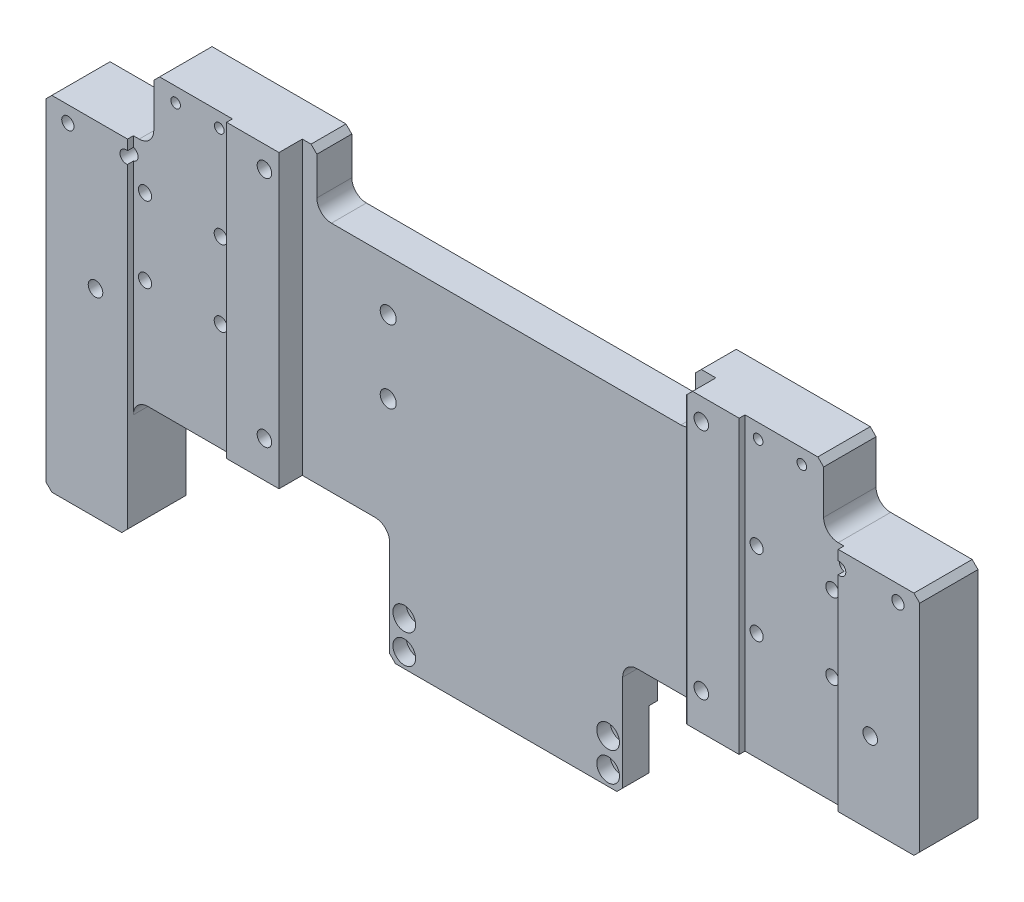
SolidWorks part; units mm, degrees
ref_plane "前视基准面" through (0, 0, 0) normal (0, 0, 1) x (1, 0, 0)
ref_plane "上视基准面" through (0, 0, 0) normal (0, 1, 0) x (1, 0, 0)
ref_plane "右视基准面" through (0, 0, 0) normal (1, 0, 0) x (0, 0, -1)
sketch "草图1" plane through (0, 0, 0) normal (0, 0, 1) x (1, 0, 0)
  line L1 (-150, -50) -> (150, -50)
  line L2 (-150, -50) -> (-150, 50)
  line L3 (-150, 50) -> (150, 50)
  line L4 (150, -50) -> (150, 50)
  line L5 (-150, -50) -> (150, 50) construction
  line L6 (-150, 50) -> (150, -50) construction
  point P0 (0, 0)
  dimension "D1" = 300
  dimension "D2" = 100
extrude "凸台-拉伸1" add sketch "草图1" along normal blind 20 contours L3 L4 L1 L2
chamfer "倒角1" distance 2 angle 45 3 edges at (-150, 50, 10) (150, 50, 10) (150, -50, 10)
sketch "草图2" plane through (0, -50, 0) normal (0, -1, 0) x (1, 0, 0)
  line L0 (-150, 20) -> (148, 20) construction
  line L1 (-122, 20) -> (-88, 20)
  line L2 (-122, 20) -> (-122, 18)
  line L3 (-122, 18) -> (-88, 18)
  line L4 (-88, 20) -> (-88, 18)
  line L6 (0, 0) -> (0, 81.6409) construction
  line L7 (88, 20) -> (88, 18)
  line L8 (122, 18) -> (88, 18)
  line L9 (122, 20) -> (122, 18)
  line L10 (122, 20) -> (88, 20)
  line L11 (-150, 20) -> (-150, 0) construction
  dimension "D1" = 34
  dimension "D2" = 28
  dimension "D3" = 2
extrude "切除-拉伸1" cut sketch "草图2" against normal through all
sketch "草图3" plane through (0, -50, 0) normal (0, -1, 0) x (1, 0, 0)
  line L5 (-88, 20) -> (88, 20) construction
  line L6 (-70, 20) -> (70, 20)
  line L7 (-70, 20) -> (-70, 12)
  line L8 (-70, 12) -> (70, 12)
  line L9 (70, 20) -> (70, 12)
  line L10 (0, 0) -> (0, 35.5532) construction
  dimension "D2" = 140
  dimension "D3" = 8
extrude "切除-拉伸2" cut sketch "草图3" against normal through all
sketch "草图4" plane through (0, 0, 0) normal (0, 0, -1) x (-1, 0, 0)
  line L0 (150, -50) -> (-148, -50) construction
  line L1 (-40, -50) -> (40, -50)
  line L2 (-40, -50) -> (-40, -90)
  line L3 (-40, -90) -> (40, -90)
  line L4 (40, -50) -> (40, -90)
  line L5 (0, 0) -> (0, -116.0992) construction
  dimension "D1" = 80
  dimension "D2" = 40
extrude "凸台-拉伸2" add sketch "草图4" against normal up to surface (12 mm away) up to face at (0, 0, 12)
fillet "圆角1" radius 5 2 edges at (40, -50, 6) (-40, -50, 6)
sketch "草图5" plane through (40, 0, 0) normal (1, 0, 0) x (0, 0, -1)
  line L1 (-3, -90) -> (0, -90)
  line L2 (-3, -90) -> (-3, -68)
  line L3 (-3, -68) -> (0, -68)
  line L4 (0, -90) -> (0, -68)
  line L5 (0, -55) -> (0, -90) construction
  line L6 (-12, -90) -> (0, -90) construction
  dimension "D1" = 22
  dimension "D3" = 3
extrude "切除-拉伸3" cut sketch "草图5" against normal through all
chamfer "倒角2" distance 2 angle 45 2 edges at (-40, -90, 7.5) (40, -90, 7.5)
sketch "草图6" plane through (0, 0, 0) normal (0, 0, -1) x (-1, 0, 0)
  line L1 (-65, 50) -> (65, 50)
  line L2 (-65, 50) -> (-65, 30)
  line L3 (-65, 30) -> (65, 30)
  line L4 (65, 50) -> (65, 30)
  line L5 (148, 50) -> (-148, 50) construction
  point P5 (0, 50)
  dimension "D1" = 20
  dimension "D2" = 130
extrude "切除-拉伸4" cut sketch "草图6" against normal through all
fillet "圆角2" radius 5 2 edges at (65, 30, 6) (-65, 30, 6)
sketch "草图9" plane through (0, 0, 0) normal (0, 0, -1) x (-1, 0, 0)
  line L0 (150, -50) -> (45, -50) construction
  line L1 (150, -50) -> (150, 48) construction
  line L2 (0, 0) -> (0, 75.4355) construction
  point P0 (133, -22)
  point P14 (-133, -22)
  dimension "D1" = 28
  dimension "D2" = 17
hole_wizard "M6 螺纹孔1" positions "草图9" profile "草图8" tap size "M6" standard "GB" end condition through all
sketch "草图8" plane through (-133, -22, 0) normal (1, 0, 0) x (0, 1, 0)
  line L0 (0, 0) -> (0, 20)
  line L1 (0, 20) -> (2.5, 20)
  line L2 (2.5, 20) -> (2.5, 0)
  line L5 (2.5, 0) -> (0, 0)
  line L11 (0, -6.35) -> (0, 107.95) construction
  dimension "通孔螺纹孔钻头直径" = 5
  dimension "通孔螺纹孔钻头深度" = 20
cosmetic thread "孔螺纹线1" parameters "D2"=6
cosmetic thread "孔螺纹线2" parameters "D2"=6
sketch "草图10" plane through (0, 0, 0) normal (0, 0, -1) x (-1, 0, 0)
  line L0 (150, -50) -> (150, 48) construction
  line L1 (150, 50) -> (115, 50)
  line L2 (150, 50) -> (150, 28)
  line L3 (150, 28) -> (115, 28)
  line L4 (115, 50) -> (115, 28)
  line L5 (148, 50) -> (65, 50) construction
  line L6 (0, 0) -> (0, 101.2863) construction
  line L7 (-115, 50) -> (-115, 28)
  line L8 (-150, 28) -> (-115, 28)
  line L9 (-150, 50) -> (-150, 28)
  line L10 (-150, 50) -> (-115, 50)
  dimension "D1" = 35
  dimension "D2" = 22
extrude "切除-拉伸5" cut sketch "草图10" against normal through all
chamfer "倒角3" distance 2 angle 45 5 edges at (150, 28, 10) (115, 50, 9) (70, 50, 16) (-115, 50, 9) (-150, 28, 10)
fillet "圆角3" radius 5 2 edges at (115, 28, 9) (-115, 28, 9)
sketch "草图13" plane through (0, 0, 0) normal (0, 0, -1) x (-1, 0, 0)
  point P0 (40.5, 12.5)
  point P3 (40.5, -12.5)
hole_wizard "M5 六角圆柱头螺钉的柱形沉头孔1" positions "草图13" profile "草图12" counterbore size "M5" standard "GB" end condition through all
sketch "草图12" plane through (-40.5, 12.5, 0) normal (1, 0, 0) x (0, 1, 0)
  line L0 (0, 0) -> (0, 20)
  line L1 (0, 20) -> (2.75, 20)
  line L3 (2.75, 20) -> (2.75, 5.7)
  line L4 (2.75, 5.7) -> (5, 5.7)
  line L5 (5, 5.7) -> (5, 0)
  line L7 (5, 0) -> (0, 0)
  line L11 (0, -6.35) -> (0, 107.95) construction
  dimension "通孔孔直径" = 5.5
  dimension "通孔孔深度" = 20
  dimension "柱形沉头孔直径" = 10
  dimension "柱形沉头孔深度" = 5.7
sketch "草图16" plane through (0, 0, 0) normal (0, 0, -1) x (-1, 0, 0)
  line L0 (0, 0) -> (0, 67.4868) construction
  point P0 (92, 13)
  point P3 (118, 13)
  point P6 (118, -13)
  point P9 (92, -13)
  point P19 (-92, -13)
  point P20 (-118, -13)
  point P21 (-118, 13)
  point P22 (-92, 13)
hole_wizard "M4 六角圆柱头螺钉的柱形沉头孔1" positions "草图16" profile "草图15" counterbore size "M4" standard "GB" end condition through all
sketch "草图15" plane through (-92, 13, 0) normal (1, 0, 0) x (0, 1, 0)
  line L0 (0, 0) -> (0, 20)
  line L1 (0, 20) -> (2.25, 20)
  line L3 (2.25, 20) -> (2.25, 4.6)
  line L4 (2.25, 4.6) -> (4, 4.6)
  line L5 (4, 4.6) -> (4, 0)
  line L7 (4, 0) -> (0, 0)
  line L11 (0, -6.35) -> (0, 107.95) construction
  dimension "通孔孔直径" = 4.5
  dimension "通孔孔深度" = 20
  dimension "柱形沉头孔直径" = 8
  dimension "柱形沉头孔深度" = 4.6
sketch "草图19" plane through (0, 0, 0) normal (0, 0, -1) x (-1, 0, 0)
  line L0 (0, 0) -> (0, 54.9806) construction
  point P0 (75, 42.5)
  point P3 (75, -37.5)
  point P12 (-75, -37.5)
  point P13 (-75, 42.5)
hole_wizard "M6 螺纹孔2" positions "草图19" profile "草图18" tap size "M6" standard "GB" end condition through all
sketch "草图18" plane through (-75, 42.5, 0) normal (1, 0, 0) x (0, 1, 0)
  line L0 (0, 0) -> (0, 20)
  line L1 (0, 20) -> (2.5, 20)
  line L2 (2.5, 20) -> (2.5, 0)
  line L5 (2.5, 0) -> (0, 0)
  line L11 (0, -6.35) -> (0, 107.95) construction
  dimension "通孔螺纹孔钻头直径" = 5
  dimension "通孔螺纹孔钻头深度" = 20
cosmetic thread "孔螺纹线3" parameters "D2"=6
cosmetic thread "孔螺纹线4" parameters "D2"=6
cosmetic thread "孔螺纹线5" parameters "D2"=6
cosmetic thread "孔螺纹线6" parameters "D2"=6
sketch "草图22" plane through (0, 0, 0) normal (0, 0, -1) x (-1, 0, 0)
  line L0 (0, 0) -> (0, 50.8482) construction
  point P0 (19.5, 20)
  point P3 (19.5, -10)
  point P11 (-19.5, -10)
  point P12 (-19.5, 20)
hole_wizard "M3 螺纹孔1" positions "草图22" profile "草图21" tap size "M3" standard "GB"
sketch "草图21" plane through (-19.5, 20, 0) normal (1, 0, 0) x (0, 1, 0)
  line L0 (0, 0) -> (0, 8.2511)
  line L1 (0, 8.2511) -> (1.25, 7.5)
  line L2 (1.25, 7.5) -> (1.25, 0)
  line L5 (1.25, 0) -> (0, 0)
  line L10 (0, 8.2511) -> (-1.25, 7.5) construction
  line L11 (0, -6.35) -> (0, 107.95) construction
  dimension "螺纹孔钻头直径" = 2.5
  dimension "螺纹孔钻头深度" = 7.5
  dimension "导头角度" = 118
cosmetic thread "孔螺纹线7" parameters "D1"=6, "D2"=3
cosmetic thread "孔螺纹线8" parameters "D1"=6, "D2"=3
cosmetic thread "孔螺纹线9" parameters "D1"=6, "D2"=3
cosmetic thread "孔螺纹线10" parameters "D1"=6, "D2"=3
sketch "草图25" plane through (0, 0, 0) normal (0, 0, -1) x (-1, 0, 0)
  line L0 (0, 0) -> (0, 56.662) construction
  point P0 (-142.5, 22.5)
  point P3 (-122.5, 22.5)
  point P12 (122.5, 22.5)
  point P13 (142.5, 22.5)
hole_wizard "M5 螺纹孔1" positions "草图25" profile "草图24" tap size "M5" standard "GB" end condition through all
sketch "草图24" plane through (142.5, 22.5, 0) normal (1, 0, 0) x (0, 1, 0)
  line L0 (0, 0) -> (0, 20)
  line L1 (0, 20) -> (2.1, 20)
  line L2 (2.1, 20) -> (2.1, 0)
  line L5 (2.1, 0) -> (0, 0)
  line L11 (0, -6.35) -> (0, 107.95) construction
  dimension "通孔螺纹孔钻头直径" = 4.2
  dimension "通孔螺纹孔钻头深度" = 20
cosmetic thread "孔螺纹线11" parameters "D2"=5
cosmetic thread "孔螺纹线12" parameters "D2"=5
cosmetic thread "孔螺纹线13" parameters "D2"=5
cosmetic thread "孔螺纹线14" parameters "D2"=5
sketch "草图30" plane through (0, 0, 12) normal (0, 0, 1) x (1, 0, 0)
  point P0 (-35, -75)
  point P3 (-35, -85)
  point P6 (35, -75)
  point P9 (35, -85)
hole_wizard "M4 六角圆柱头螺钉的柱形沉头孔3" positions "草图30" profile "草图27" counterbore size "M4" standard "GB" end condition through all
sketch "草图27" plane through (-35, -75, 12) normal (1, 0, 0) x (0, -1, 0)
  line L0 (0, 0) -> (0, 12)
  line L1 (0, 12) -> (2.25, 12)
  line L3 (2.25, 12) -> (2.25, 4.6)
  line L4 (2.25, 4.6) -> (3.9, 4.6)
  line L5 (3.9, 4.6) -> (3.9, 0)
  line L7 (3.9, 0) -> (0, 0)
  line L11 (0, -6.35) -> (0, 107.95) construction
  dimension "通孔孔直径" = 4.5
  dimension "通孔孔深度" = 12
  dimension "柱形沉头孔直径" = 7.8
  dimension "柱形沉头孔深度" = 4.6
chamfer "倒角4" distance 2 angle 45 2 edges at (65, 50, 6) (-65, 50, 6)
sketch "草图31" plane through (0, -50, 0) normal (0, -1, 0) x (1, 0, 0)
  line L0 (-150, 0) -> (-45, 0) construction
  line L1 (-150, 20) -> (-122, 20)
  line L2 (-150, 20) -> (-150, 0)
  line L3 (-150, 0) -> (-122, 0)
  line L4 (-122, 20) -> (-122, 0)
extrude "凸台-拉伸3" add sketch "草图31" along normal blind 40
chamfer "倒角5" distance 2 angle 45 2 edges at (-150, -90, 10) (-122, -90, 10)
fillet "圆角4" radius 5 1 edges at (-122, -50, 9)
sketch "草图34" plane through (0, 0, 0) normal (0, 0, -1) x (-1, 0, 0)
  point P0 (-107.5, 45)
  point P3 (-92.5, 45)
  point P6 (92.5, 45)
  point P9 (107.5, 45)
hole_wizard "M4 螺纹孔1" positions "草图34" profile "草图33" tap size "M4" standard "GB" end condition through all
sketch "草图33" plane through (107.5, 45, 0) normal (1, 0, 0) x (0, 1, 0)
  line L0 (0, 0) -> (0, 20)
  line L1 (0, 20) -> (1.65, 20)
  line L2 (1.65, 20) -> (1.65, 0)
  line L5 (1.65, 0) -> (0, 0)
  line L11 (0, -6.35) -> (0, 107.95) construction
  dimension "通孔螺纹孔钻头直径" = 3.3
  dimension "通孔螺纹孔钻头深度" = 20
cosmetic thread "孔螺纹线15" parameters "D2"=4
cosmetic thread "孔螺纹线16" parameters "D2"=4
cosmetic thread "孔螺纹线17" parameters "D2"=4
cosmetic thread "孔螺纹线18" parameters "D2"=4
